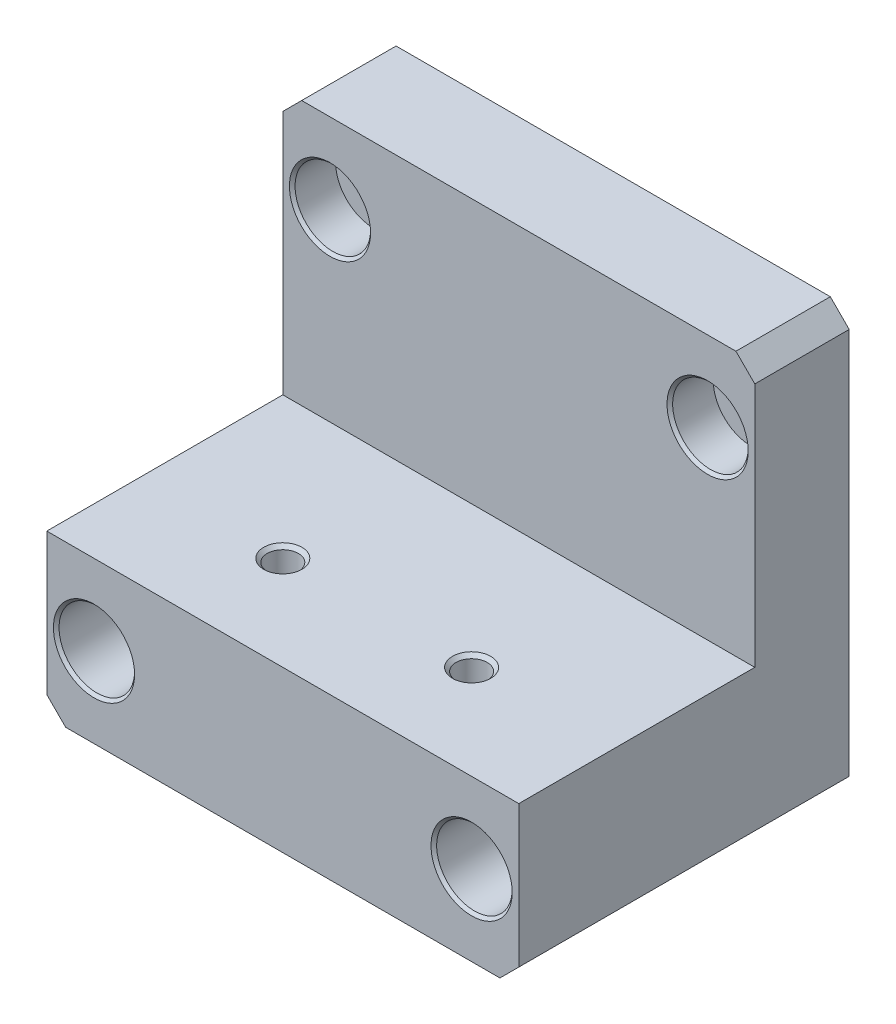
SolidWorks part; units mm, degrees
ref_plane "前视基准面" through (0, 0, 0) normal (0, 0, 1) x (1, 0, 0)
ref_plane "上视基准面" through (0, 0, 0) normal (0, 1, 0) x (1, 0, 0)
ref_plane "右视基准面" through (0, 0, 0) normal (1, 0, 0) x (0, 0, -1)
sketch "草图1" plane through (0, 0, 0) normal (0, 0, 1) x (1, 0, 0)
  line L1 (0, 0) -> (-50, 0)
  line L2 (0, 0) -> (0, 45)
  line L3 (0, 45) -> (-50, 45)
  line L4 (-50, 0) -> (-50, 45)
  dimension "D1" = 50
  dimension "D2" = 45
extrude "凸台-拉伸1" add sketch "草图1" along normal blind 10
sketch "草图6" plane through (0, 0, 10) normal (0, 0, 1) x (1, 0, 0)
  line L0 (-50, 45) -> (-50, 0) construction
  line L1 (-50, 17) -> (0, 17)
  line L2 (-50, 17) -> (-50, 0)
  line L3 (-50, 0) -> (0, 0)
  line L4 (0, 17) -> (0, 0)
  dimension "D1" = 17
extrude "凸台-拉伸2" add sketch "草图6" along normal blind 25
chamfer "倒角1" distance 2 angle 45 4 edges at (0, 0, 17.5) (-50, 0, 17.5) (0, 45, 5) (-50, 45, 5)
hole_wizard "打孔尺寸(%根据)内六角圆柱头螺钉的类型1" positions "草图5" profile "草图4" counterbore size "M4" standard "GB"
sketch "草图5" plane through (0, 0, 10) normal (0, 0, 1) x (1, 0, 0)
  point P6 (-45, 36.5)
  point P9 (-5, 36.5)
sketch "草图4" plane through (-45, 36.5, 10) normal (1, 0, 0) x (0, -1, 0)
  line L0 (0, 0) -> (0, 11.2919)
  line L1 (0, 11.2919) -> (2.15, 10)
  line L2 (2.15, 10) -> (2.15, 4.6)
  line L3 (2.15, 4.6) -> (4, 4.6)
  line L5 (4, 4.6) -> (4, 0.3)
  line L6 (4, 0.3) -> (4.3, 0)
  line L7 (4.3, 0) -> (0, 0)
  line L8 (-4, 0.3) -> (-4.3, 0) construction
  line L10 (0, 11.2919) -> (-2.15, 10) construction
  line L11 (0, -6.35) -> (0, 107.95) construction
  dimension "孔直径" = 4.3
  dimension "孔深度" = 10
  dimension "锥形沉头孔直径" = 8
  dimension "锥形沉头孔深度" = 4.6
  dimension "近端锥形沉头孔直径" = 8.6
  dimension "近端锥形沉头孔角度" = 90
  dimension "导头角度" = 118
hole_wizard "打孔尺寸(%根据)内六角圆柱头螺钉的类型2" positions "草图7" profile "草图8" counterbore size "M4" standard "GB" end condition through all
sketch "草图7" plane through (0, 0, 35) normal (0, 0, 1) x (1, 0, 0)
  line L0 (-45, 36.5) -> (-45, -3.8583) construction
  line L2 (-5, 36.5) -> (-5, -5.984) construction
  line L5 (-48, 0) -> (-2, 0) construction
  point P0 (-45, 8.5)
  point P2 (-5, 8.5)
  dimension "D1" = 8.5
sketch "草图8" plane through (-45, 8.5, 35) normal (1, 0, 0) x (0, -1, 0)
  line L0 (0, 0) -> (0, 35)
  line L1 (0, 35) -> (2.15, 35)
  line L3 (2.15, 35) -> (2.15, 25)
  line L4 (4, 25) -> (2.15, 25)
  line L5 (4, 25) -> (4, 0.3)
  line L6 (4, 0.3) -> (4.3, 0)
  line L7 (4.3, 0) -> (0, 0)
  line L8 (-4, 0.3) -> (-4.3, 0) construction
  line L11 (0, -6.35) -> (0, 107.95) construction
  dimension "通孔孔直径" = 4.3
  dimension "通孔孔深度" = 35
  dimension "柱形沉头孔直径" = 8
  dimension "柱形沉头孔深度" = 25
  dimension "近端锥形沉头孔直径" = 8.6
  dimension "近端锥形沉头孔角度" = 90
hole_wizard "M4 螺纹孔1" positions "草图9" profile "草图10" tap size "M4" standard "GB" end condition through all
sketch "草图9" plane through (0, 17, 0) normal (0, 1, 0) x (1, 0, 0)
  line L0 (-25, -35) -> (-25, -13.8779) construction
  line L1 (0, -35) -> (-50, -35) construction
  point P0 (-35, -25)
  point P2 (-15, -25)
  dimension "D1" = 20
  dimension "D2" = 10
sketch "草图10" plane through (-35, 17, 25) normal (1, 0, 0) x (0, 0, 1)
  line L0 (0, 0) -> (0, 17)
  line L1 (0, 17) -> (1.65, 17)
  line L2 (1.65, 17) -> (1.65, 0.375)
  line L3 (1.65, 0.375) -> (2.025, 0)
  line L5 (2.025, 0) -> (0, 0)
  line L6 (-1.65, 0.375) -> (-2.025, 0) construction
  line L11 (0, -6.35) -> (0, 107.95) construction
  dimension "通孔螺纹孔钻头直径" = 3.3
  dimension "通孔螺纹孔钻头深度" = 17
  dimension "近端锥形沉头孔直径" = 4.05
  dimension "近端锥形沉头孔角度" = 90
cosmetic thread "孔螺蚊线1"
cosmetic thread "孔螺蚊线2"
